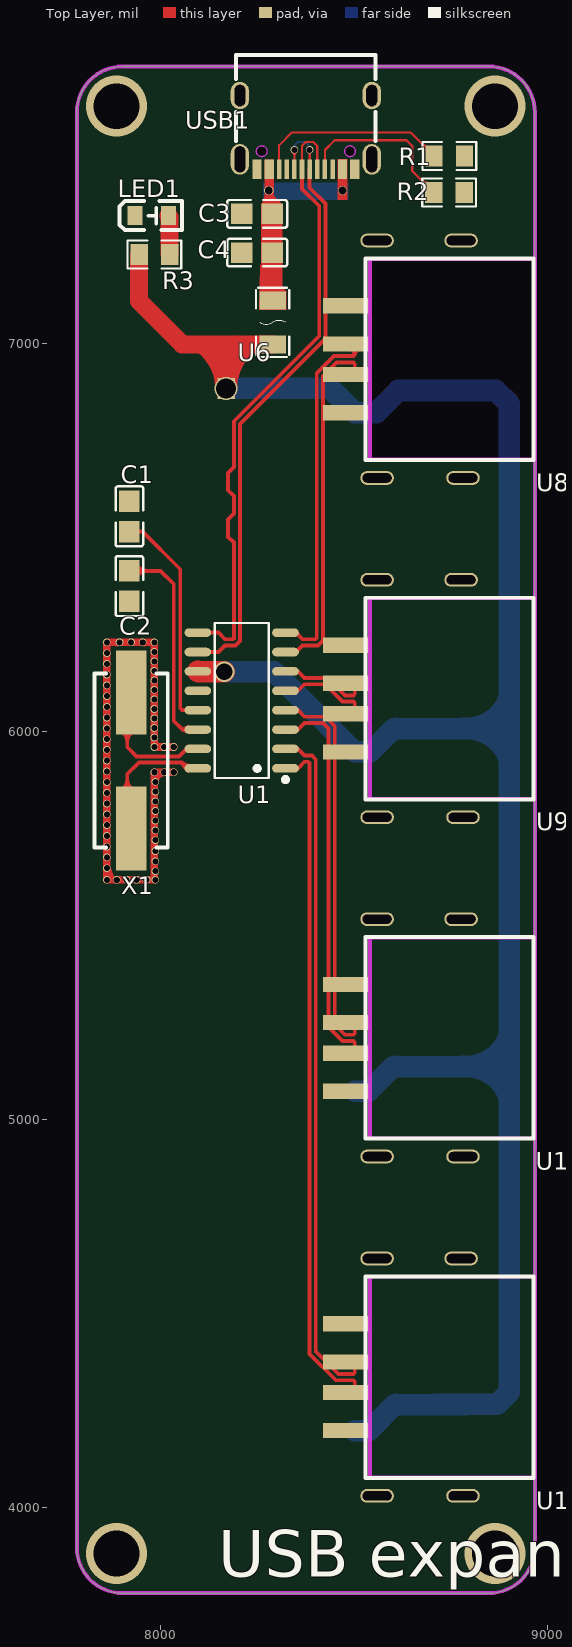
[diagram p0: Top Layer view]
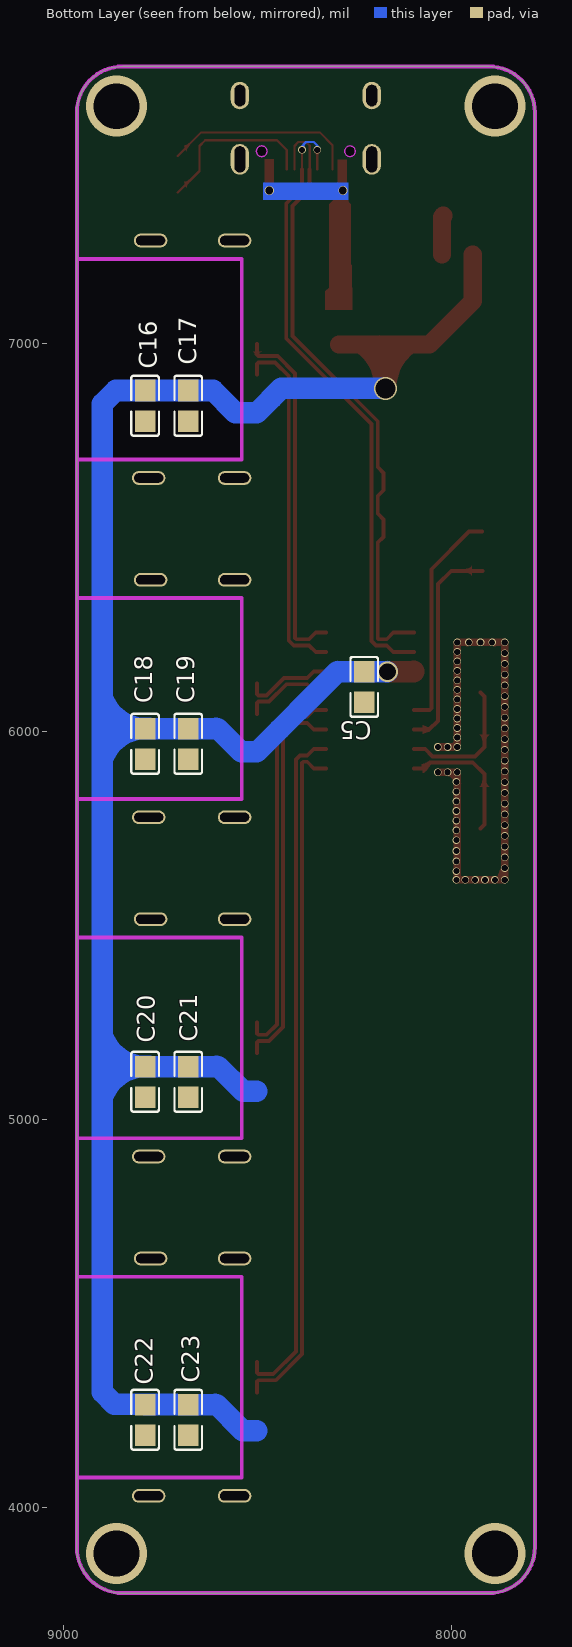
[diagram p1: Bottom Layer view, seen from below]
# Altium PCB MISC51874.pcbdoc
Units mil, origin at the board's own origin, x right, y up, seen from the top; angles counter-clockwise.
Board outline 1181.1 x 3937.01 mil, 2 copper layers (Top Layer, Bottom Layer), stack 62.206 mil thick; 25 components, 20 nets, 107 pads, 68 vias.

## Layer stack, top to bottom
Top Solder Mask Layer: solder mask 0.394, Dk 3.3
Top Layer: signal copper 1.379
Dielectric1: surface 59.449, FR4, Dk 4.5
Bottom Layer: signal copper 1.378
Bottom Solder Mask Layer: solder mask 0.394, Dk 3.3

## Board outline
7903.11,7715 ccw(c7903.11,7596.89) 7785,7596.89 7785,3896.1 ccw(c7903.11,3896.1) 7903.11,3777.99 8847.99,3777.99 ccw(c8847.99,3896.1) 8966.1,3896.1 8966.1,7596.89 ccw(c8847.99,7596.89) 8847.99,7715
cut-out: 8540.7,7218.86 8540.7,6700.16 8962.68,6700.16 8962.68,7218.86

## Design rules (kind name [scope] priority, off if disabled: settings)
BoardOutlineClearance copperThickness2oz_1 [All] p2 off: genericclearance=8 ignorepadtopadclearanceinfootprint=FALSE except(0: Arc-SplitContinuation Track-SplitContinuation SMDPad-SplitContinuation THPad-SplitContinuation Via-SplitContinuation Fill-SplitContinuation Region-SplitContinuation Poly-SplitContinuation Text-SplitContinuation Hole-SplitContinuation; 6: SMDPad-CutoutEdge THPad-CutoutEdge Via-CutoutEdge Fill-CutoutEdge Region-CutoutEdge Text-CutoutEdge Hole-CutoutEdge; 10: Poly-OutlineEdge Poly-CutoutEdge; 11.8: Arc-OutlineEdge Track-OutlineEdge SMDPad-OutlineEdge THPad-OutlineEdge Via-OutlineEdge Fill-OutlineEdge Region-OutlineEdge Text-OutlineEdge Hole-OutlineEdge Arc-CutoutEdge Track-CutoutEdge)
BoardOutlineClearance Plane_innerPlane_1 [All] p4 off: genericclearance=4 ignorepadtopadclearanceinfootprint=FALSE except(0: Arc-SplitContinuation Track-SplitContinuation SMDPad-SplitContinuation THPad-SplitContinuation Via-SplitContinuation Fill-SplitContinuation Region-SplitContinuation Poly-SplitContinuation Text-SplitContinuation Hole-SplitContinuation; 6: SMDPad-CutoutEdge THPad-CutoutEdge Via-CutoutEdge Fill-CutoutEdge Region-CutoutEdge Text-CutoutEdge Hole-CutoutEdge; 10: Poly-OutlineEdge Poly-CutoutEdge; 11.8: Arc-OutlineEdge Track-OutlineEdge SMDPad-OutlineEdge THPad-OutlineEdge Via-OutlineEdge Fill-OutlineEdge Region-OutlineEdge Text-OutlineEdge Hole-OutlineEdge Arc-CutoutEdge Track-CutoutEdge)
BoardOutlineClearance Copper_copperRegion_1 [All] p6 off: genericclearance=4 ignorepadtopadclearanceinfootprint=FALSE except(0: Arc-SplitContinuation Track-SplitContinuation SMDPad-SplitContinuation THPad-SplitContinuation Via-SplitContinuation Fill-SplitContinuation Region-SplitContinuation Poly-SplitContinuation Text-SplitContinuation Hole-SplitContinuation; 6: SMDPad-CutoutEdge THPad-CutoutEdge Via-CutoutEdge Fill-CutoutEdge Region-CutoutEdge Text-CutoutEdge Hole-CutoutEdge; 10: Poly-OutlineEdge Poly-CutoutEdge; 11.8: Arc-OutlineEdge Track-OutlineEdge SMDPad-OutlineEdge THPad-OutlineEdge Via-OutlineEdge Fill-OutlineEdge Region-OutlineEdge Text-OutlineEdge Hole-OutlineEdge Arc-CutoutEdge Track-CutoutEdge)
BoardOutlineClearance copperThickness1oz_1 [All] p8: genericclearance=4 ignorepadtopadclearanceinfootprint=FALSE except(0: Arc-SplitContinuation Track-SplitContinuation SMDPad-SplitContinuation THPad-SplitContinuation Via-SplitContinuation Fill-SplitContinuation Region-SplitContinuation Poly-SplitContinuation Text-SplitContinuation Hole-SplitContinuation; 6: SMDPad-CutoutEdge THPad-CutoutEdge Via-CutoutEdge Fill-CutoutEdge Region-CutoutEdge Text-CutoutEdge Hole-CutoutEdge; 10: Poly-OutlineEdge Poly-CutoutEdge; 11.8: Arc-OutlineEdge Track-OutlineEdge SMDPad-OutlineEdge THPad-OutlineEdge Via-OutlineEdge Fill-OutlineEdge Region-OutlineEdge Text-OutlineEdge Hole-OutlineEdge Arc-CutoutEdge Track-CutoutEdge)
Clearance copperThickness2oz [All] p1 off: gap=8 ignorepadtopadclearanceinfootprint=FALSE except(6: SMDPad-Track SMDPad-SMDPad THPad-Track SMDPad-THPad THPad-THPad Track-Via SMDPad-Via THPad-Via Via-Via Fill-Track Region-Track Fill-SMDPad Region-SMDPad Fill-THPad Region-THPad Fill-Via Region-Via Fill-Fill Fill-Region Region-Region Arc-Track Arc-SMDPad Arc-THPad Arc-Via Fill-Arc Region-Arc Arc-Arc Text-Track SMDPad-Text Text-THPad Text-Via Fill-Text Region-Text Arc-Text Text-Text Hole-Track Hole-SMDPad Hole-THPad Hole-Via Fill-Hole Region-Hole Hole-Arc Hole-Text; 10: Poly-Track Poly-SMDPad Poly-THPad Poly-Via Poly-Fill Poly-Region Poly-Poly Poly-Arc Poly-Text Poly-Hole)
Clearance Plane_innerPlane [All] p3 off: gap=4 ignorepadtopadclearanceinfootprint=FALSE except(6: SMDPad-Track SMDPad-SMDPad THPad-Track SMDPad-THPad THPad-THPad Track-Via SMDPad-Via THPad-Via Via-Via Fill-Track Region-Track Fill-SMDPad Region-SMDPad Fill-THPad Region-THPad Fill-Via Region-Via Fill-Fill Fill-Region Region-Region Arc-Track Arc-SMDPad Arc-THPad Arc-Via Fill-Arc Region-Arc Arc-Arc Text-Track SMDPad-Text Text-THPad Text-Via Fill-Text Region-Text Arc-Text Text-Text Hole-Track Hole-SMDPad Hole-THPad Hole-Via Fill-Hole Region-Hole Hole-Arc Hole-Text; 10: Poly-Track Poly-SMDPad Poly-THPad Poly-Via Poly-Fill Poly-Region Poly-Poly Poly-Arc Poly-Text Poly-Hole)
Clearance Copper_copperRegion [All] p5 off: gap=4 ignorepadtopadclearanceinfootprint=FALSE except(6: SMDPad-Track SMDPad-SMDPad THPad-Track SMDPad-THPad THPad-THPad Track-Via SMDPad-Via THPad-Via Via-Via Fill-Track Region-Track Fill-SMDPad Region-SMDPad Fill-THPad Region-THPad Fill-Via Region-Via Fill-Fill Fill-Region Region-Region Arc-Track Arc-SMDPad Arc-THPad Arc-Via Fill-Arc Region-Arc Arc-Arc Text-Track SMDPad-Text Text-THPad Text-Via Fill-Text Region-Text Arc-Text Text-Text Hole-Track Hole-SMDPad Hole-THPad Hole-Via Fill-Hole Region-Hole Hole-Arc Hole-Text; 10: Poly-Track Poly-SMDPad Poly-THPad Poly-Via Poly-Fill Poly-Region Poly-Poly Poly-Arc Poly-Text Poly-Hole)
Clearance copperThickness1oz [All] p7: gap=4 ignorepadtopadclearanceinfootprint=FALSE except(6: SMDPad-Track SMDPad-SMDPad THPad-Track SMDPad-THPad THPad-THPad Track-Via SMDPad-Via THPad-Via Via-Via Fill-Track Region-Track Fill-SMDPad Region-SMDPad Fill-THPad Region-THPad Fill-Via Region-Via Fill-Fill Fill-Region Region-Region Arc-Track Arc-SMDPad Arc-THPad Arc-Via Fill-Arc Region-Arc Arc-Arc Text-Track SMDPad-Text Text-THPad Text-Via Fill-Text Region-Text Arc-Text Text-Text Hole-Track Hole-SMDPad Hole-THPad Hole-Via Fill-Hole Region-Hole Hole-Arc Hole-Text; 10: Poly-Track Poly-SMDPad Poly-THPad Poly-Via Poly-Fill Poly-Region Poly-Poly Poly-Arc Poly-Text Poly-Hole)
DiffPairsRouting differentialPair [All] p1: maxlimit=6 minlimit=6 mostfreqgap=6 toplayer_minwidth=5 toplayer_prefwidth=10 toplayer_maxwidth=100 toplayer_mingap=6 toplayer_prefgap=6 toplayer_maxgap=6 bottomlayer_minwidth=5 bottomlayer_prefwidth=10 bottomlayer_maxwidth=100 bottomlayer_mingap=6 bottomlayer_prefgap=6 bottomlayer_maxgap=6 maxuncoupledlength=5
HoleToHoleClearance otherClearance [All] p1: gap=11.8 allowstackedmicrovias=TRUE
Length netLength [All] p1: minlimit=0 maxlimit=0
PasteMaskExpansion pasteMaskExpansion [All] p1: expansion=0
PlaneConnect innerPlane [All] p1: planeconnectstyle=Relief reliefexpansion=20 reliefentries=4 reliefconductorwidth=10 reliefairgap=10
PolygonConnect copperRegion [All] p1: connectstyle=Relief reliefconductorwidth=10 reliefentries=4 polygonreliefangle="90 Angle" airgapwidth=10 via.connectstyle=Relief via.reliefconductorwidth=10 via.reliefentries=4 via.polygonreliefangle="90 Angle" via.airgapwidth=10
RoutingVias viaSize [All] p1: holewidth=12 width=24 viastyle="Through Hole" minholewidth=11.8 minwidth=19.7 maxholewidth=248 maxwidth=393.7
SolderMaskExpansion solderMaskExpansion [IsVia] p1: expansion=-1000 istentingtop=TRUE
SolderMaskExpansion solderMaskExpansion [All] p2: expansion=2 istentingtop=FALSE
Width copperThickness2oz_2 [All] p1 off: maxlimit=100 minlimit=8 preferedwidth=10
Width copperThickness1oz_2 [All] p2: maxlimit=100 minlimit=5 preferedwidth=10

## Components (designator, comment, footprint, x,y, rotation, side; value= is the part's Value field where it differs from the comment)
C1 "100nF" C0805 7920.55,6554.77 r90 top
C2 "100nF" C0805 7920.55,6375 r270 top
C3 "10UF" C0805 8250,7335 r0 top
C4 "0.1UF" C0805 8250,7235 r0 top
C5 "0.1UF" C0805 8225,6115 r90 bottom
C16 "10UF" C0805 8790,6840 r90 bottom
C17 "0.1UF" C0805 8678.82,6840 r90 bottom
C18 "10UF" C0805 8790,5968.33 r90 bottom
C19 "0.1UF" C0805 8678.82,5968.36 r90 bottom
C20 "10UF" C0805 8790,5096.67 r90 bottom
C21 "0.1UF" C0805 8678.82,5096.71 r90 bottom
C22 "10UF" C0805 8790,4225 r90 bottom
C23 "0.1UF" C0805 8678.82,4225.07 r90 bottom
LED1 "" LED_0805 7980,7330 r0 top
R1 "5.1K" R0805 8745.6,7484.04 r0 top
R2 "5.1K" R0805 8745,7390 r0 top
R3 "2K" R0805 7985,7230 r180 top
U1 "SL2.1A" SOP-16_L10.0-W3.9-P1.27-LS6.0-BL 8210,6080 r90 top
U6 "1.5A快恢复保险丝-1206" F1206 8290,7055 r270 top
U8 "USB-A-018" usb-smd_usb-a-018 8630,6960 r90 top
U9 "USB-A-018" usb-smd_usb-a-018 8630,6085 r90 top
U10 "USB-A-018" usb-smd_usb-a-018 8630,5210 r90 top
U11 "USB-A-018" usb-smd_usb-a-018 8630,4335 r90 top
USB1 "typec" USB-C-SMD_KH-TYPE-C-16P 8375.55,7545 r180 top
X1 "12MHz" CRYSTAL-SMD_L11.1-W4.8-LS12.3 7925,5925 r270 top

## Footprints (in the part's own frame and the unit in brackets; to place one, negate y for a bottom-side part, rotate by r counter-clockwise, add the part's x,y. Pads: shape width x height; smd on the part's side, far side on the other; paste and mask are expansions set on the pad)
C0805 [mm]
  rect 1.41x1.35 smd paste-100 mask+0.051: 1(-1,0) 2(1,0)
  silkscreen extent -1.96,-0.9 1.96,0.9
CRYSTAL-SMD_L11.1-W4.8-LS12.3 [mm]
  rect 5.5x2 smd: 1(-4.45,0) 2(4.45,0)
  silkscreen extent -5.7,-2.4 5.7,2.4
F1206 [mm]
  rect 1.19x1.728 smd: 1(-1.445,0) 2(1.445,0)
  silkscreen extent -2.27,-1.09 2.27,1.09
LED_0805 [mm]
  rect 1x1.25 smd paste+0 mask+0.051: 1(-1.15,0.005) 2(1.05,0.005)
  silkscreen extent -2.15,-0.94 1.93,0.97
R0805 [mm]
  rect 1.133x1.377 smd paste-100 mask+0.051: 1(-1,0) 2(1,0)
  silkscreen extent -1.76,-0.92 1.76,0.92
SOP-16_L10.0-W3.9-P1.27-LS6.0-BL [mm]
  oval 0.56x1.745 smd: 1(-4.445,-2.872) 2(-3.175,-2.872) 3(-1.905,-2.872) 4(-0.635,-2.872) 5(0.635,-2.872) 6(1.905,-2.872) 7(3.175,-2.872) 8(4.445,-2.872) 9(4.445,2.872) 10(3.175,2.872) 11(1.905,2.872) 12(0.635,2.872) 13(-0.635,2.872) 14(-1.905,2.872) 15(-3.175,2.872) 16(-4.445,2.872)
  silkscreen extent -5.33,-3.02 5.08,1.77
USB-C-SMD_KH-TYPE-C-16P [mm]
  oval 1.2x2 hole 0.7 slot 1.7 at 90 deg: 1(-4.32,1.765) 2(4.32,1.765)
  oval 1.2x1.8 hole 0.7 slot 1.4 at 90 deg: 3(-4.32,-2.415) 4(4.32,-2.415)
  rect 0.3x1.3 smd paste-100 mask+0.05: A1(-3.35,2.415) A4(-2.55,2.415) A5(-1.25,2.415) A6(-0.25,2.415) A7(0.25,2.415) A8(1.25,2.415) A9(2.55,2.415) A12(3.35,2.415) B1(3.05,2.415) B4(2.25,2.415) B5(1.75,2.415) B6(0.75,2.415) B7(-0.75,2.415) B8(-1.75,2.415) B9(-2.25,2.415) B12(-3.05,2.415)
  Board Outline Layer circle w0.003: c-2.89,1.235 r0.35
  Board Outline Layer circle w0.003: c2.89,1.235 r0.35
  Board Outline Layer region: -3.24,1.235 -3.205,1.387 -3.108,1.509 -2.968,1.576 -2.812,1.576 -2.672,1.509 -2.575,1.387 -2.54,1.235 -2.54,1.235 -2.575,1.083 -2.672,0.961 -2.812,0.894 -2.968,0.894 -3.108,0.961 -3.205,1.083 -3.24,1.235
  Board Outline Layer region: -3.24,1.235 -3.231,1.313 -3.205,1.387 -3.164,1.453 -3.108,1.509 -3.042,1.55 -2.968,1.576 -2.89,1.585 -2.812,1.576 -2.738,1.55 -2.672,1.509 -2.616,1.453 -2.575,1.387 -2.549,1.313 -2.54,1.235 -2.549,1.157 -2.575,1.083 -2.616,1.017 -2.672,0.961 -2.738,0.92 -2.812,0.894 -2.89,0.885 -2.968,0.894 -3.042,0.92 -3.108,0.961 -3.164,1.017 -3.205,1.083 -3.231,1.157
  Board Outline Layer region: 2.54,1.235 2.575,1.387 2.672,1.509 2.812,1.576 2.968,1.576 3.108,1.509 3.205,1.387 3.24,1.235 3.24,1.235 3.205,1.083 3.108,0.961 2.968,0.894 2.812,0.894 2.672,0.961 2.575,1.083 2.54,1.235
  Board Outline Layer region: 2.54,1.235 2.549,1.313 2.575,1.387 2.616,1.453 2.672,1.509 2.738,1.55 2.812,1.576 2.89,1.585 2.968,1.576 3.042,1.55 3.108,1.509 3.164,1.453 3.205,1.387 3.231,1.313 3.24,1.235 3.231,1.157 3.205,1.083 3.164,1.017 3.108,0.961 3.042,0.92 2.968,0.894 2.89,0.885 2.812,0.894 2.738,0.92 2.672,0.961 2.616,1.017 2.575,1.083 2.549,1.157
  Multi-Layer board cut-out: -3.24,1.235 -3.205,1.387 -3.108,1.509 -2.968,1.576 -2.812,1.576 -2.672,1.509 -2.575,1.387 -2.54,1.235 -2.54,1.235 -2.575,1.083 -2.672,0.961 -2.812,0.894 -2.968,0.894 -3.108,0.961 -3.205,1.083 -3.24,1.235
  Multi-Layer board cut-out: 2.54,1.235 2.575,1.387 2.672,1.509 2.812,1.576 2.968,1.576 3.108,1.509 3.205,1.387 3.24,1.235 3.24,1.235 3.205,1.083 3.108,0.961 2.968,0.894 2.812,0.894 2.672,0.961 2.575,1.083 2.54,1.235
  silkscreen extent -4.57,-5.08 4.57,0.57
usb-smd_usb-a-018 [mm]
  rect 1x3 smd paste-100 mask+0.05: 1(-3.5,3.832) 2(-1,3.832) 3(1,3.832) 4(3.5,3.832)
  oval 0.9x2.2 hole 0.6 slot 1.9 at 90 deg paste+0 mask+0.05: 5(-7.775,1.795) 6(7.775,1.795) 7(7.775,-3.705) 8(-7.775,-3.832)
  Board Outline Layer lines w0.254: -4.47,2.268 6.575,2.268 6.575,-8.482 ; -4.375,2.268 -6.575,2.268 -6.575,-8.482
  silkscreen extent -6.6,-8.45 6.6,2.55

## Free pads (board coordinates)
  rect 44.59x54.21 smd paste-3937.01 mask+2: 17(8170,6885)

## Via types
v1: diameter 19.68, hole 15.7, Top Layer to Bottom Layer, 60 vias
v2: diameter 157.48, hole 118.1, Top Layer to Bottom Layer, 4 vias
v3: diameter 23.62, hole 19.7, Top Layer to Bottom Layer, 2 vias
v4: diameter 53.15, hole 43.3, Top Layer to Bottom Layer, 1 vias
v5: diameter 59.06, hole 51.2, Top Layer to Bottom Layer, 1 vias

## Nets (pads, with @x,y where several pads share a name; then routed paths per layer and width w, separated by ;. In a path a pad name is that pad's centre, name@x,y a point inside that pad or via, vN(x,y) a via of type N, cw(c..) or ccw(c..) an arc to the next point about the centre after c; other vN are vias at no path point)
$1N748: C2.1 U1.14 | length 552.9
  Top Layer w10: C2.1@7920,6414.37 8000.63,6414.37 8035,6380 8035,6027.56 8057.56,6005 U1.14
$1N752: C1.1 U1.13 | length 576.5
  Top Layer w10: C1.1@7921.09,6515.4 7954.6,6515.4 8051.56,6418.44 8051.56,6060 8056.56,6055 U1.13
$1N850: U1.15 X1.1 | length 344.1
  Top Layer w10: X1.1 7915,6090.2 7915,5960 7939,5936 8048.57,5936 8067.57,5955 U1.15
$1N854: U1.16 X1.2 | length 344.9
  Top Layer w10: X1.2 7915,5759.8 7915,5890 7945,5920 8055,5920 8070,5905 U1.16
$1N2453: LED1.2 R3.1 | length 101.5
  Top Layer w46.85: LED1.2 8024.37,7327.17 R3.1
+5V: C5.2 C16.2 C17.2 C18.2 C19.2 C20.2 C21.2 C22.2 C23.2 pad.17 R3.2 U1.11 U6.2 U8.1 U9.1 U10.1 U11.1 | length 5738.3
  Top Layer w46.85: R3.2 7945,7229.37 7945,7110 8056.89,6998.11 U6.2
  Top Layer w55.51: U1.11 8097.54,6154.37 v4(8165,6154.37) ; v5(8170,6885) 8170,6990
  Bottom Layer w55.51: v4(8165,6154.37) C5.2 8294.5,6154.37 8501.66,5947.21 8542.21,5947.21 8602.73,6007.73 C19.2 C18.2 ; v5(8170,6885) 8438.86,6885 8501.66,6822.21 8557.21,6822.21 8614.37,6879.37 C17.2 C16.2 8865.63,6879.37 8900,6845 8900,6006.95 ; 8501.66,4197.21 8537.77,4197.21 8605,4264.44 C23.2 C22.2@8789.93,4264.44 ; 8501.66,5072.21 8537.21,5072.21 8601.08,5136.08 C21.2 8790,5136.08 8899.55,5136.08 8900,5136.53 ; C22.2 8790.63,4265 8869.14,4265 8900,4295.86 8900,5136.53 ; C18.2 8899.25,6007.7 8900,6006.95 ; 8900,5136.53 8900,6006.95
CC1: R2.1 USB1.A5 | length 434.8
  Top Layer w5.71: USB1.A5 8424.76,7499.76 8450,7525 8635,7525 8650,7510 8650,7445.63 R2.1
CC2: R1.1 USB1.B5 | length 500.4
  Top Layer w5.71: USB1.B5 8306.65,7511.65 8340,7545 8645.27,7545 R1.1
DM: U1.9 USB1.A7 USB1.B7 | length 1613.4
  Top Layer w5.71: USB1.A7 8365.71,7510.71 8375,7520 8395,7520 8405,7510 8405,7450 USB1.B7
  Top Layer w10: U1.9 8150,6255 8167.01,6237.99 8187.99,6237.99 8190,6240 8190,6487.03 8175,6502.03 8175,6547.03 8190,6562.03 8190,6607.03 8175,6622.03 8175,6667.03 8190,6682.03 8190,6800 8410,7020 8410,7355 8365.71,7399.29 USB1.A7
DM1: U1.7 U8.2 U9.2 U10.2 U11.2 | length 916.8
  Top Layer w10: U1.7 8350,6205 8367.01,6222.01 8406.63,6222.02 8419.53,6234.91 8419.53,6916.9 8454.64,6952.01 8498.12,6952.01 8501.66,6948.47 U8.2@8501.66,6920.63
DM2: U1.5 | length 233.6
  Top Layer w10: U1.5 8355,6105 8372.01,6122.01 8425.28,6122.01 8470.28,6077.01 8498.12,6077.01 8501.66,6073.47 8501.66,6045.63
DM3: U1.3 | length 1005.5
  Top Layer w10: U1.3 8355,6005 8372.01,6022.01 8420,6022.01 8434,6008.01 8434,5238.28 8470.28,5202.01 8498.12,5202.01 8501.66,5198.47 8501.66,5170.63
DM4: U1.1 | length 1768
  Top Layer w10: U1.1 8355,5905 8372.01,5922.01 8381.46,5922.01 8385,5918.47 8385,4395 8452.99,4327.01 8498.12,4327.01 8501.66,4323.47 8501.66,4295.63
DP: U1.10 USB1.A6 USB1.B6 | length 1616
  Top Layer w5.71: v1@8340,7500 8346.02,7493.98 USB1.B6 ; USB1.A6 v1(8385.39,7500)
  Top Layer w10: U1.10 8150,6205 8167.01,6222.01 8194.61,6222.01 8205.98,6233.38 8205.98,6793.38 8425.98,7013.38 8425.98,7361.64 8385.39,7402.24 USB1.A6
  Bottom Layer w5.71: v1(8346.02,7500) 8346.02,7511.02 8355,7520 8375,7520 8385.39,7509.61 v1(8385.39,7500)
DP1: U1.8 U8.3 U9.3 U10.3 U11.3 | length 916.8
  Top Layer w10: U1.8 8350,6255 8366.99,6238.01 8400.01,6238 8403.54,6241.54 8403.54,6923.54 8447.99,6967.99 8498.12,6967.99 8501.66,6971.53 U8.3@8501.66,6999.37
DP2: U1.6 | length 233.6
  Top Layer w10: U1.6 8355,6155 8372.01,6137.99 8432.01,6137.99 8477.01,6092.99 8498.12,6092.99 8501.66,6096.53 8501.66,6124.37
DP3: U1.4 | length 1005.5
  Top Layer w10: U1.4 8355,6055 8372.01,6037.99 8426.62,6037.99 8450,6014.61 8450,5244.91 8476.92,5217.99 8498.12,5217.99 8501.66,5221.53 8501.66,5249.37
DP4: U1.2 | length 1769.7
  Top Layer w10: U1.2 8355,5955 8372.01,5937.99 8391,5937.99 8401,5927.99 8401,4401.63 8459.64,4342.99 8498.12,4342.99 8501.66,4346.53 8501.66,4374.37
GND: C1.2 C2.2 C3.1 C4.1 C5.1 C16.1 C17.1 C18.1 C19.1 C20.1 C21.1 C22.1 C23.1 LED1.1 R1.2 R2.2 U1.12 U8.4 U8.5 U8.6 U8.7 U8.8 U9.4 U9.5 U9.6 U9.7 U9.8 U10.4 U10.5 U10.6 U10.7 U10.8 U11.4 U11.5 U11.6 U11.7 U11.8 USB1.1 USB1.2 USB1.3 USB1.4 USB1.A1 USB1.A12 USB1.B1 USB1.B12 | length 1502.7
  Top Layer w19.68: v1(8035,5895) v1(8010,5895) v1(7985,5895) 7985,5620 v1(7987.5,5617.5) v1(7964.5,5617.5) v1(7939,5617.5) v1(7913.5,5617.5) v1(7888,5617.5) v1(7862.5,5617.5) v1(7862.5,5647.73) v1(7862.5,5675.45) v1(7862.5,5703.18) v1(7862.5,5730.91) v1(7862.5,5758.64) v1(7862.5,5786.36) v1(7862.5,5814.09) v1(7862.5,5841.82) v1(7862.5,5869.55) v1(7862.5,5897.27) v1(7862.5,5925) v1(7862.5,5952.73) v1(7862.5,5980.45) v1(7862.5,6008.18) v1(7862.5,6035.91) v1(7862.5,6063.64) v1(7862.5,6091.36) v1(7862.5,6119.09) v1(7862.5,6146.82) v1(7862.5,6174.55) v1(7862.5,6202.27) v1(7862.5,6230) v1(7895,6230) v1(7925,6230) v1(7955,6230) v1(7985,6230) v1(7985,6205.45) v1(7985,6180.91) v1(7985,6156.36) v1(7985,6131.82) v1(7985,6107.27) v1(7985,6082.73) v1(7985,6058.18) v1(7985,6033.64) v1(7985,6009.09) v1(7985,5984.55) 7985,5970 7995,5960 v1(8010,5960) v1(8035,5960)
  other v1: 7987.5,5640 7987.5,5665 7987.5,5692.04 7987.5,5720 7987.5,5745 7987.5,5770 7987.5,5795 7987.5,5820 7987.5,5845 7987.5,5870 7985,5960
VCC+5V: C3.2 C4.2 U6.1 USB1.A4 USB1.A9 USB1.B4 USB1.B9
  other v3: 8280,7395 8470,7395
pads on no net: USB1.A8 USB1.B8
copper on no net:
  other v2: 7887.36,3880.35 8863.74,3880.35 7887.36,7612.64 8863.74,7612.64

## Polygon pours and split planes (outlines as drawn)
GND on Top Layer (solid, remove dead copper, pour order 0): 3000,7840 3000,3155 5140,3155 5140,7840
GND on Bottom Layer (solid, remove dead copper, pour order 4): 4615,7610 4615,3000 6710,3000 6710,7610

## Keep-outs
Board Outline Layer:
  region: 8540.7,7218.86 8540.7,6700.16 8962.68,6700.16 8962.68,7218.86
  region: 8540.7,7218.86 8540.7,6700.16 8962.68,6700.16 8962.68,7218.86
  lines w0.1: 8540.7,6700.16 8540.7,7218.86 8962.68,7218.86 8962.68,6700.16 8540.7,6700.16
  lines w10: 7785,3896.1 7785,7596.89 cw(c7903.11,7596.89) 7903.11,7715 8847.99,7715 cw(c8847.99,7596.89) 8966.1,7596.89 8966.1,3896.1 cw(c8847.99,3896.1) 8847.99,3777.99 7903.11,3777.99 cw(c7903.11,3896.1) 7785,3896.1

## Other copper
Top Layer:
  region net VCC+5V: 8270,7475 8292.87,7475 8292.87,7382.13 8315,7360 8315,7145 8325,7135 8325,7086.98 8256,7086.98 8257.72,7202.72 8260,7205 8260,7360 8265,7365 8270,7381.46
  region net VCC+5V: 8458.44,7475.51 8481.85,7475.51 8481.85,7371.7 8458.44,7371.7
  region net DP1: 8496.66,6971.53 8506.66,6971.53 8507.01,6973.93 8508.06,6976.12 8509.7,6977.9 8511.79,6979.13 8514.16,6979.69 8489.16,6979.69 8491.52,6979.13 8493.61,6977.9 8495.25,6976.12 8496.3,6973.93 8496.66,6971.53
  region net GND: 7994.84,5865.47 7994.9,5867.32 7995.09,5869.14 7995.4,5870.94 7995.83,5872.7 7996.38,5874.4 7997.04,5876.03 7997.83,5877.57 7998.73,5879.01 7999.75,5880.33 8000.3,5880.94 8000.88,5881.52 8001.49,5882.07 8002.12,5882.57 8002.79,5883.04 8003.48,5883.47 8004.2,5883.85 8004.95,5884.18 8005.72,5884.47 8006.52,5884.72 8007.35,5884.91 8008.21,5885.04 8009.09,5885.13 8010,5885.16 8010,5904.84 7994.84,5895 7975.16,5865.47
  region net GND: 7872.34,5647.03 7852.66,5647.03 7862.5,5627.34 7888,5607.66
  region net GND: 7892.03,6220.16 7882.19,6239.84 7877.83,6239.51 7873.58,6238.52 7869.53,6236.89 7872.34,6223.11 7878.8,6221.48 7885.38,6220.49 7892.03,6220.16
  region net GND: 7965.31,6239.84 7955.47,6220.16 7962.12,6220.49 7968.7,6221.48 7975.16,6223.11 7977.97,6236.89 7973.92,6238.52 7969.67,6239.51 7965.31,6239.84
  region net $1N854: 8058.54,5923.54 8051.96,5915.97 8053.02,5914.82 8054.73,5912.69 8061.22,5903.82 8064.05,5900.3 8065.5,5898.71 8066.96,5897.28 8068.43,5896.06 8069.17,5895.53 8069.91,5895.08 8070.65,5894.7 8071.38,5894.39 8072.12,5894.16 8072.85,5894.02 8073.58,5893.98 8076.65,5916.02 8075.62,5916.07 8074.5,5916.19 8073.33,5916.39 8071.49,5916.83 8069.58,5917.41 8067.65,5918.11 8065.75,5918.92 8063.92,5919.81 8062.2,5920.78 8060.65,5921.79 8059.72,5922.48 8058.9,5923.18
  region net $1N854: 7920,5873.07 7910,5873.07 7909.68,5869.61 7908.72,5866.27 7907.17,5863.17 7905.07,5860.4 7902.5,5858.07 7927.5,5858.07 7924.93,5860.4 7922.83,5863.17 7921.28,5866.27 7920.32,5869.61 7920,5873.07
  region net $1N748: 8057.56,6010 8057.56,6000 8058.49,5999.74 8070.8,5994.92 8072.65,5994.24 8073.58,5993.98 8073.58,6016.02 8072.65,6015.76 8060.34,6010.94 8058.49,6010.26
  region net $1N748: 7962.12,6409.37 7962.12,6419.37 7958.66,6419.69 7955.33,6420.65 7952.22,6422.2 7949.45,6424.3 7947.12,6426.87 7947.12,6401.87 7949.45,6404.44 7952.22,6406.54 7955.33,6408.09 7958.66,6409.05 7962.12,6409.37
  region net $1N850: 7910,5976.93 7920,5976.93 7920.32,5980.39 7921.28,5983.73 7922.83,5986.83 7924.93,5989.6 7927.5,5991.93 7902.5,5991.93 7905.07,5989.6 7907.17,5986.83 7908.72,5983.73 7909.68,5980.39 7910,5976.93
  region net CC2: 8677.88,7516.43 8677.88,7508.36 8680.11,7505.74 8681.89,7502.79 8683.17,7499.6 8683.93,7496.25 8689.21,7511.15 8686.07,7511.7 8683.08,7512.79 8680.32,7514.38 8677.88,7516.43
  region net CC1: 8677.28,7422.39 8677.28,7414.31 8679.51,7411.69 8681.29,7408.75 8682.58,7405.56 8683.34,7402.2 8688.62,7417.11 8685.48,7417.66 8682.48,7418.75 8679.72,7420.34 8677.28,7422.39
  region net DP: 8343.17,7486.6 8348.88,7486.6 8348.9,7487.21 8348.98,7487.77 8349.1,7488.29 8349.26,7488.76 8349.47,7489.2 8349.71,7489.61 8349.99,7489.99 8350.29,7490.37 8350.98,7491.08 8352.56,7492.6 8353.4,7493.49 8338.64,7493.49 8339.48,7492.6 8341.07,7491.08 8341.75,7490.37 8342.06,7489.99 8342.33,7489.61 8342.57,7489.2 8342.78,7488.76 8342.94,7488.29 8343.07,7487.77 8343.14,7487.21
  region net +5V: 8185.71,7021.54 8185.71,6974.68 8199.93,6975.08 8214.12,6976.24 8228.22,6978.19 8242.18,6980.91 8255.98,6984.38 8255.98,7011.84 8242.18,7015.31 8228.22,7018.03 8214.12,7019.98 8199.93,7021.14 8185.71,7021.54
  region net +5V: 8197.76,6885 8142.24,6885 8141.87,6894.31 8140.75,6903.57 8138.88,6912.7 8136.29,6921.66 8132.99,6930.37 8128.99,6938.8 8124.34,6946.87 8119.04,6954.55 8113.15,6961.77 8106.7,6968.5 8099.72,6974.68 8240.28,6974.68 8233.3,6968.5 8226.85,6961.77 8220.96,6954.55 8215.66,6946.87 8211.01,6938.8 8207.01,6930.37 8203.71,6921.66 8201.12,6912.7 8199.25,6903.57 8198.13,6894.31
Bottom Layer:
  region net VCC+5V: 8265.8,7415.02 8485,7415.02 8485,7371.7 8265.8,7371.7
  region net +5V: 8680.16,6907.13 8680.16,6851.61 8694.21,6851.94 8708.23,6852.9 8722.19,6854.5 8736.06,6856.74 8749.81,6859.61 8763.42,6863.11 8763.42,6895.63 8749.81,6899.13 8736.06,6902 8722.19,6904.24 8708.23,6905.84 8694.21,6906.8 8680.16,6907.13
  region net +5V: 8788.66,6851.61 8788.66,6907.13 8747.03,6907.21 8705.39,6907.47 8705.39,6907.13 8705.39,6851.61 8705.39,6851.27 8747.03,6851.53 8788.66,6851.61
  region net +5V: 8865.63,6851.61 8865.63,6907.13 8857.17,6906.8 8848.75,6905.83 8840.44,6904.21 8832.27,6901.97 8824.3,6899.1 8816.58,6895.63 8816.58,6863.11 8824.3,6859.64 8832.27,6856.77 8840.44,6854.53 8848.75,6852.91 8857.17,6851.94 8865.63,6851.61
  region net +5V: 8788.66,4236.68 8788.66,4292.2 8747.03,4292.28 8705.39,4292.54 8705.39,4292.2 8705.39,4236.68 8705.39,4236.34 8747.03,4236.6 8788.66,4236.68
  region net +5V: 8865.63,6851.61 8865.63,6907.13 8857.17,6906.8 8848.75,6905.83 8840.44,6904.21 8832.27,6901.97 8824.3,6899.1 8816.58,6895.63 8816.58,6863.11 8824.3,6859.64 8832.27,6856.77 8840.44,6854.53 8848.75,6852.91 8857.17,6851.94 8865.63,6851.61
  region net +5V: 8865.63,6851.61 8865.63,6907.13 8857.17,6906.8 8848.75,6905.83 8840.44,6904.21 8832.27,6901.97 8824.3,6899.1 8816.58,6895.63 8816.58,6863.11 8824.3,6859.64 8832.27,6856.77 8840.44,6854.53 8848.75,6852.91 8857.17,6851.94 8865.63,6851.61
  region net +5V: 8165,6182.13 8165,6126.61 8170.99,6126.94 8176.9,6127.93 8182.67,6129.57 8188.23,6131.83 8193.5,6134.69 8198.42,6138.11 8198.42,6170.63 8193.5,6174.05 8188.23,6176.91 8182.67,6179.17 8176.9,6180.81 8170.99,6181.8
  region net +5V: 8788.66,5979.97 8788.66,6035.48 8774.61,6035.16 8760.59,6034.2 8746.63,6032.6 8732.76,6030.36 8719,6027.49 8705.39,6023.99 8705.39,5991.46 8719,5987.97 8732.76,5985.1 8746.63,5982.86 8760.59,5981.25 8774.61,5980.29 8788.66,5979.97
  region net +5V: 8899.25,5979.95 8899.25,6035.46 8885.3,6035.14 8871.37,6034.18 8857.51,6032.57 8843.74,6030.33 8830.08,6027.46 8816.58,6023.97 8816.58,5991.44 8830.08,5987.94 8843.74,5985.07 8857.51,5982.83 8871.37,5981.23 8885.3,5980.27 8899.25,5979.95
  region net +5V: 8865.63,6851.61 8865.63,6907.13 8857.17,6906.8 8848.75,6905.83 8840.44,6904.21 8832.27,6901.97 8824.3,6899.1 8816.58,6895.63 8816.58,6863.11 8824.3,6859.64 8832.27,6856.77 8840.44,6854.53 8848.75,6852.91 8857.17,6851.94 8865.63,6851.61
  region net +5V: 8788.66,5108.33 8788.66,5163.84 8774.61,5163.52 8760.59,5162.56 8746.63,5160.95 8732.76,5158.71 8719,5155.84 8705.39,5152.35 8705.39,5119.82 8719,5116.32 8732.76,5113.45 8746.63,5111.21 8760.59,5109.61 8774.61,5108.65 8788.66,5108.33
  region net +5V: 8790,5108.33 8790,5163.84 8798.09,5164.21 8806.11,5165.31 8814,5167.15 8821.69,5169.69 8829.11,5172.93 8836.21,5176.83 8842.92,5181.36 8849.19,5186.48 8854.96,5192.15 8860.2,5198.33 8864.85,5204.96 8868.88,5211.99 8872.24,5219.35 8872.24,5052.82 8868.88,5060.18 8864.85,5067.2 8860.2,5073.83 8854.96,5080.01 8849.19,5085.69 8842.92,5090.81 8836.21,5095.34 8829.11,5099.24 8821.69,5102.47 8814,5105.02 8806.11,5106.85 8798.09,5107.96
  region net +5V: 8899.25,5979.95 8899.25,6035.46 8885.3,6035.14 8871.37,6034.18 8857.51,6032.57 8843.74,6030.33 8830.08,6027.46 8816.58,6023.97 8816.58,5991.44 8830.08,5987.94 8843.74,5985.07 8857.51,5982.83 8871.37,5981.23 8885.3,5980.27 8899.25,5979.95
  region net +5V: 8790,5979.95 8790,6035.46 8798.09,6035.83 8806.11,6036.93 8814,6038.77 8821.69,6041.31 8829.11,6044.55 8836.21,6048.45 8842.92,6052.98 8849.19,6058.1 8854.96,6063.78 8860.2,6069.95 8864.85,6076.58 8868.88,6083.61 8872.24,6090.97 8872.24,5924.44 8868.88,5931.8 8864.85,5938.82 8860.2,5945.45 8854.96,5951.63 8849.19,5957.31 8842.92,5962.43 8836.21,5966.96 8829.11,5970.86 8821.69,5974.09 8814,5976.64 8806.11,5978.47 8798.09,5979.58
  region net +5V: 8605,4292.2 8605,4236.68 8613.17,4237.01 8621.29,4237.98 8629.31,4239.6 8637.17,4241.85 8644.83,4244.71 8652.24,4248.18 8652.24,4280.7 8644.83,4284.17 8637.17,4287.03 8629.31,4289.28 8621.29,4290.9 8613.17,4291.87
  region net +5V: 8601.08,5163.84 8601.08,5108.33 8609.89,5108.65 8618.64,5109.62 8627.3,5111.24 8635.82,5113.48 8644.15,5116.35 8652.24,5119.82 8652.24,5152.35 8644.15,5155.82 8635.82,5158.68 8627.3,5160.93 8618.64,5162.54 8609.89,5163.51 8601.08,5163.84
  region net +5V: 8602.73,6035.48 8602.73,5979.97 8611.26,5980.3 8619.75,5981.27 8628.14,5982.88 8636.38,5985.13 8644.43,5987.99 8652.24,5991.46 8652.24,6023.99 8644.43,6027.46 8636.38,6030.33 8628.14,6032.57 8619.75,6034.19 8611.26,6035.16 8602.73,6035.48
  region net +5V: 8614.37,6907.13 8614.37,6851.61 8621.05,6851.94 8627.67,6852.92 8634.16,6854.55 8640.46,6856.81 8646.5,6859.67 8652.24,6863.11 8652.24,6895.63 8646.5,6899.07 8640.46,6901.93 8634.16,6904.19 8627.67,6905.82 8621.05,6906.8 8614.37,6907.13
  region net DP: 8348.88,7511.02 8343.17,7511.02 8343.02,7510.39 8342.62,7509.77 8342.03,7509.18 8341.33,7508.61 8339.16,7507 8338.64,7506.51 8353.4,7506.51 8352.88,7507 8350.71,7508.61 8350.01,7509.18 8349.42,7509.77 8349.02,7510.39
  region net DP: 8382.74,7516.3 8378.7,7512.26 8379.16,7511.66 8379.43,7511.01 8379.51,7510.32 8379.45,7509.57 8379.26,7508.79 8378.97,7507.98 8378.17,7506.29 8376.79,7503.65 8376.37,7502.77 8376.02,7501.9 8375.75,7501.04 8375.59,7500.2 8375.57,7499.38 8386.01,7509.82 8385.26,7510.08 8384.74,7510.66 8384.38,7511.5 8383.89,7513.55 8383.62,7514.6 8383.26,7515.55
  region net +5V: 8294.5,6126.61 8294.5,6182.13 8287.01,6181.8 8279.59,6180.82 8272.28,6179.2 8265.14,6176.95 8258.22,6174.09 8251.58,6170.63 8251.58,6138.11 8258.22,6134.65 8265.14,6131.79 8272.28,6129.54 8279.59,6127.92 8287.01,6126.94 8294.5,6126.61
  region net +5V: 8462.4,6025.72 8423.15,5986.46 8482.03,5966.84 8542.21,5919.45
  region net +5V: 8473.9,6889.22 8442.78,6841.84 8448.24,6836.85 8454.13,6832.39 8460.41,6828.49 8467.02,6825.18 8473.9,6822.49 8501.38,6849.96 8497.01,6858.55 8492.05,6866.8 8486.53,6874.69 8480.47,6882.18 8473.9,6889.22

## Silkscreen, mask and mechanical layers (free items; w line width, h text height)
Top Silkscreen Layer:
  text "USB expansion dock" at 8150,3820 h120
Mechanical Layer:
  lines w0.1: 8540.7,6700.16 8540.7,7218.86 8962.68,7218.86 8962.68,6700.16 8540.7,6700.16